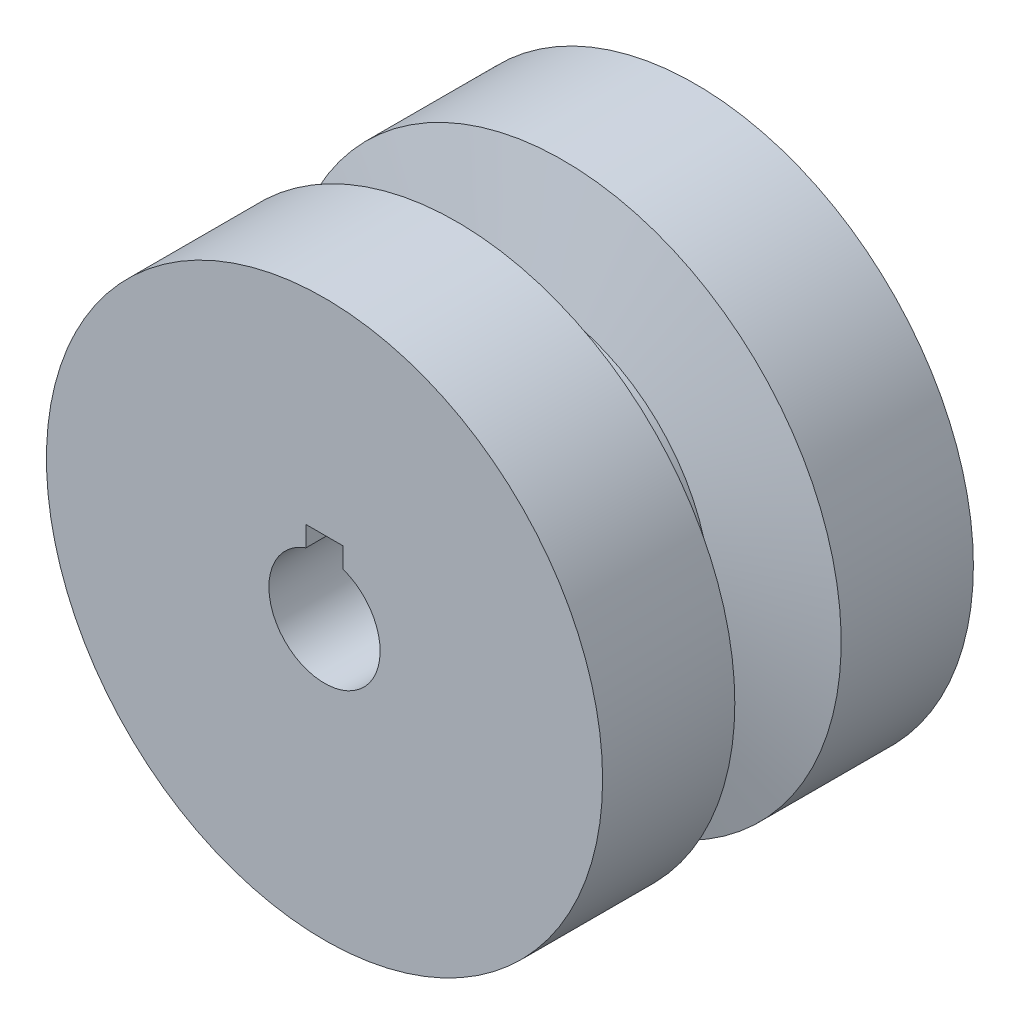
SolidWorks part; units mm, degrees
material "普通碳钢"
ref_plane "前视基准面" through (0, 0, 0) normal (0, 0, 1) x (1, 0, 0)
ref_plane "上视基准面" through (0, 0, 0) normal (0, 1, 0) x (1, 0, 0)
ref_plane "右视基准面" through (0, 0, 0) normal (1, 0, 0) x (0, 0, -1)
sketch "草图1" plane through (0, 0, 0) normal (0, 0, 1) x (1, 0, 0)
  circle A0 centre (0, 0) radius 37.5
  circle A1 centre (0, 0) radius 7.5
  dimension "D1" = 75
  dimension "D2" = 15
extrude "凸台-拉伸1" add sketch "草图1" along normal blind 50
sketch "草图2" plane through (0, 0, 0) normal (0, 1, 0) x (1, 0, 0)
  line L0 (37.5, -25) -> (-44.7851, -25) construction
  line L1 (37.5, -50) -> (37.5, 0) construction
  line L2 (0, 0) -> (0, -52.3687) construction
  line L3 (-38.25, -17.6488) -> (-23.25, -21.25)
  line L4 (-23.25, -21.25) -> (-23.25, -28.75)
  line L5 (-38.25, -17.6488) -> (-38.25, -32.3512)
  line L6 (-38.25, -32.3512) -> (-23.25, -28.75)
  point P11 (-23.25, -25)
  point P13 (-38.25, -25)
  dimension "D1" = 23.25
  dimension "D2" = 3.75
  dimension "D3" = 13.5
  dimension "D4" = 15
revolve "切除-旋转1" cut sketch "草图2" angle 360 about L2
ref_plane "基准面1" through (0, 32.5, 0) normal (0, 1, 0) x (1, 0, 0)
hole_wizard "M5 螺纹孔2" positions "草图4" profile "草图3" tap size "M5" standard "Iso"
sketch "草图4" plane through (0, 32.5, 0) normal (0, 1, 0) x (1, 0, 0)
  line L0 (0, 0) -> (0, -9)
  point P2 (0, -9)
  dimension "D1" = 9
sketch "草图3" plane through (0, 32.5, 9) normal (1, 0, 0) x (0, 0, 1)
  line L0 (0, 0) -> (0, 31.2618)
  line L1 (0, 31.2618) -> (2.1, 30)
  line L2 (2.1, 30) -> (2.1, 0)
  line L5 (2.1, 0) -> (0, 0)
  line L10 (0, 31.2618) -> (-2.1, 30) construction
  line L11 (0, -6.35) -> (0, 107.95) construction
  dimension "螺纹孔钻头直径" = 4.2
  dimension "螺纹孔钻头深度" = 30
  dimension "导头角度" = 118
cosmetic thread "孔螺蚊线1" parameters "D1"=22.7, "D2"=6
ref_plane "基准面2" through (32.5, 0, 0) normal (1, 0, 0) x (0, 0, -1)
hole_wizard "M5 螺纹孔1" positions "草图6" profile "草图5" tap size "M5" standard "Iso"
sketch "草图6" plane through (32.5, 0, 0) normal (1, 0, 0) x (0, 0, -1)
  line L0 (0, 0) -> (-9, 0)
  point P2 (-9, 0)
  dimension "D1" = 9
sketch "草图5" plane through (32.5, 0, 9) normal (0, 1, 0) x (0, 0, -1)
  line L0 (0, 0) -> (0, 31.2618)
  line L1 (0, 31.2618) -> (2.1, 30)
  line L2 (2.1, 30) -> (2.1, 0)
  line L5 (2.1, 0) -> (0, 0)
  line L10 (0, 31.2618) -> (-2.1, 30) construction
  line L11 (0, -6.35) -> (0, 107.95) construction
  dimension "螺纹孔钻头直径" = 4.2
  dimension "螺纹孔钻头深度" = 30
  dimension "导头角度" = 118
cosmetic thread "孔螺蚊线2" parameters "D1"=25, "D2"=5
sketch "草图7" plane through (0, 0, 0) normal (0, 0, -1) x (-1, 0, 0)
  line L0 (0, 0) -> (0, 38.7676) construction
  line L1 (-2.5, 5.2) -> (2.5, 5.2)
  line L2 (-2.5, 5.2) -> (-2.5, 9.8)
  line L3 (-2.5, 9.8) -> (2.5, 9.8)
  line L4 (2.5, 5.2) -> (2.5, 9.8)
  line L5 (-2.5, 5.2) -> (2.5, 9.8) construction
  line L6 (-2.5, 9.8) -> (2.5, 5.2) construction
  circle A0 centre (0, 0) radius 7.5 construction
  point P0 (0, 7.5)
  dimension "D1" = 5
  dimension "D2" = 4.6
extrude "切除-拉伸1" cut sketch "草图7" against normal blind 90
